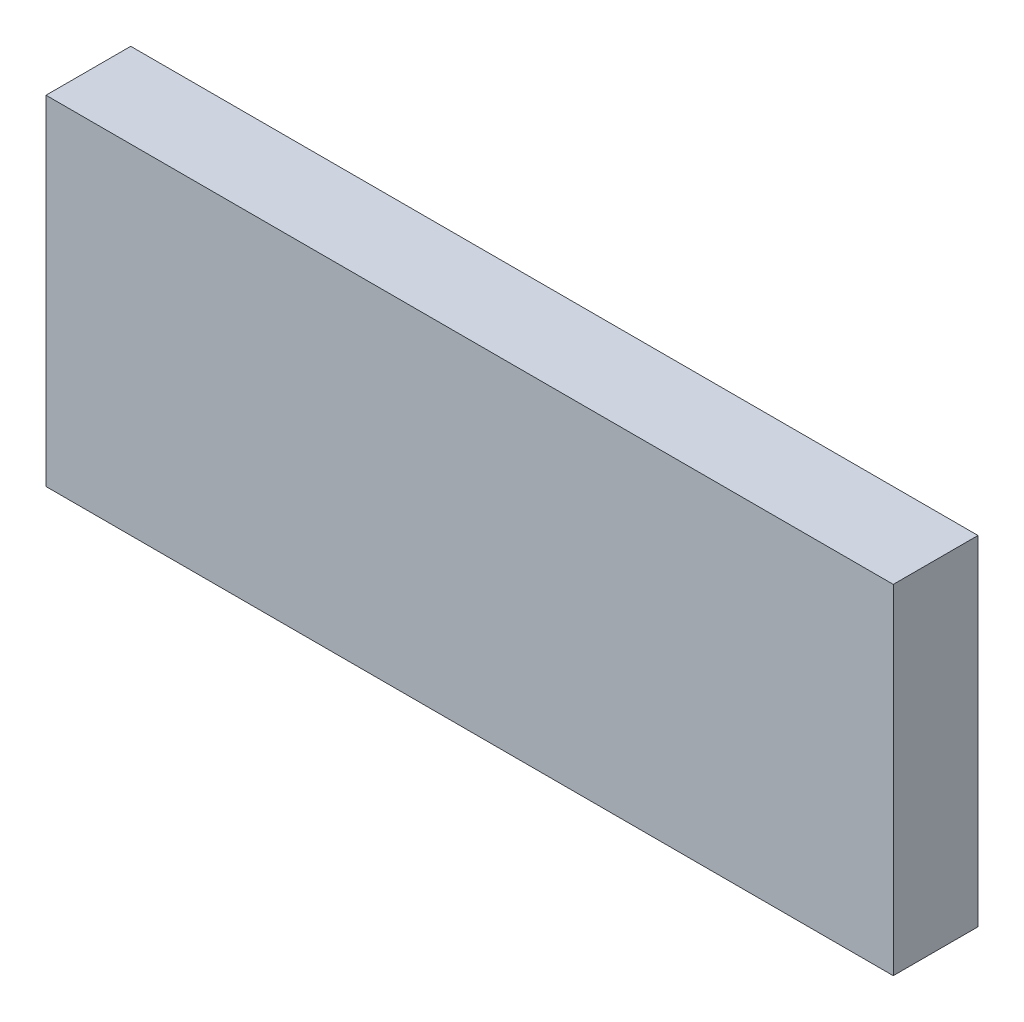
SolidWorks part; units mm, degrees
ref_plane "Front Plane" through (0, 0, 0) normal (0, 0, 1) x (1, 0, 0)
ref_plane "Top Plane" through (0, 0, 0) normal (0, 1, 0) x (1, 0, 0)
ref_plane "Right Plane" through (0, 0, 0) normal (1, 0, 0) x (0, 0, -1)
sketch "Sketch1" plane through (0, 0, 0) normal (0, 0, 1) x (1, 0, 0)
  line L1 (0, 0) -> (-250, 0)
  line L2 (0, 0) -> (0, 100)
  line L3 (0, 100) -> (-250, 100)
  line L4 (-250, 0) -> (-250, 100)
  dimension "D1" = 250
  dimension "D2" = 100
extrude "Boss-Extrude1" add sketch "Sketch1" along normal blind 25
